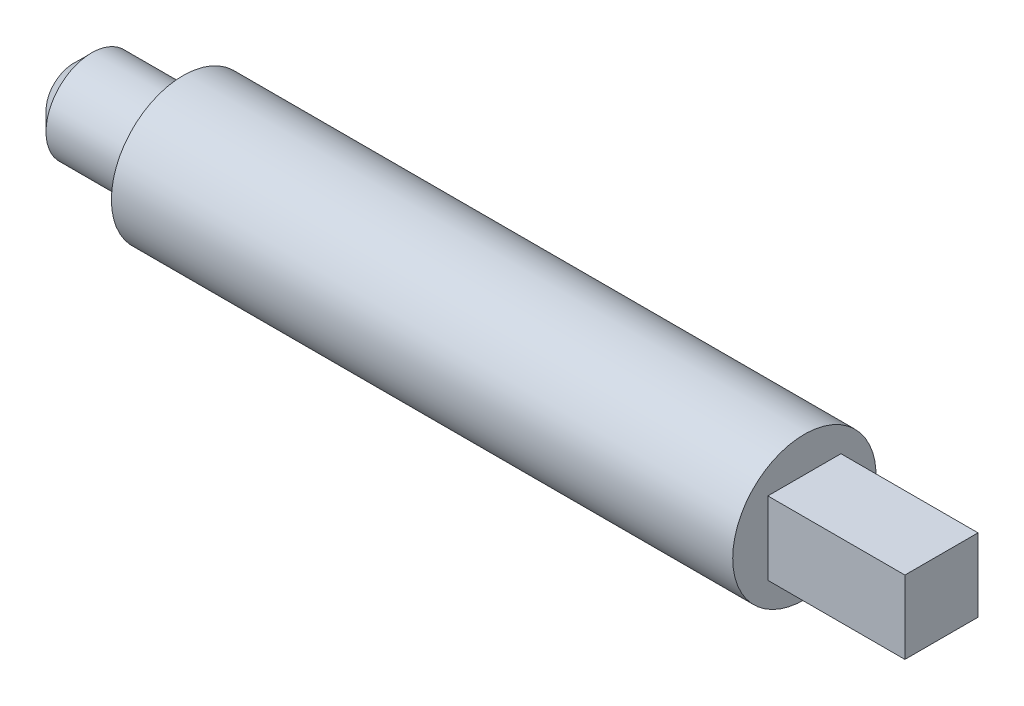
from build123d import *

# Parameters (mm, degrees)
SKETCH2_W           = 8
SKETCH2_H           = 8
BOSS_EXTRUDE1_DEPTH = 15
CHAMFER1_SIZE       = 2


with BuildPart() as part:
    # Sketch1 → Revolve1 (revolve)
    with BuildSketch(Plane.XY, mode=Mode.PRIVATE) as revolve1_sk:
        Polygon((0, 0), (0, 5), (12, 5), (12, 7.845), (80, 7.845), (80, 0), align=None)
    revolve(revolve1_sk.sketch.rotate(Axis((0, 0, 0), (1, 0, 0)), 90), axis=Axis((0, 0, 0), (1, 0, 0)))

    # Sketch2 → Boss-Extrude1 (add)
    with BuildSketch(Plane(origin=(80, 0, 0), x_dir=(0, 0, -1), z_dir=(1, 0, 0))):
        Rectangle(SKETCH2_W, SKETCH2_H)
    extrude(amount=BOSS_EXTRUDE1_DEPTH)

    # Chamfer1
    chamfer1_edges = [part.edges().sort_by_distance(p)[0] for p in [
        (0, 0, -5),
    ]]
    chamfer(chamfer1_edges, length=CHAMFER1_SIZE)


solid = part.part
